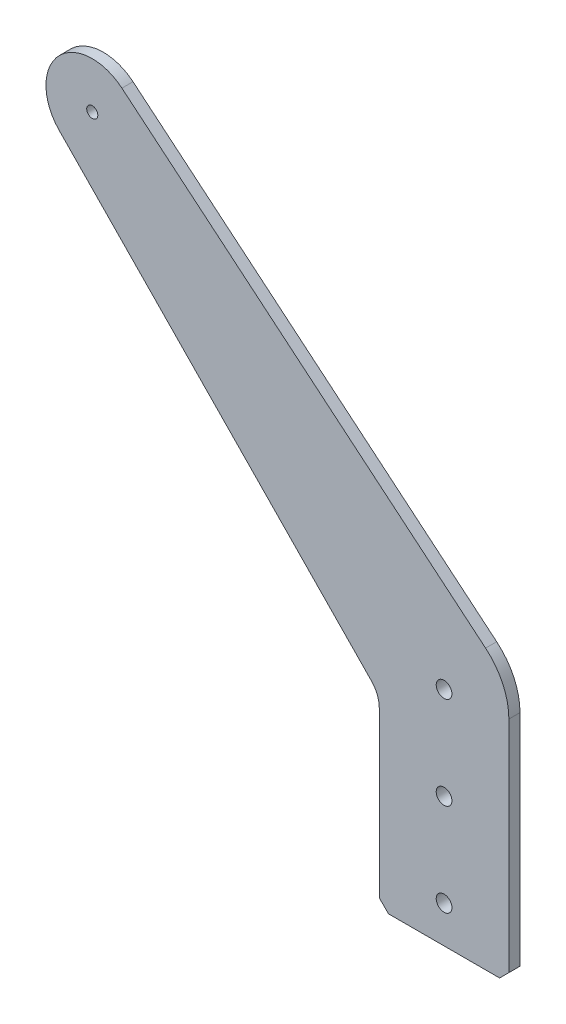
from build123d import *

# Parameters (mm, degrees)
SKETCH_1_R      = 3
SKETCH_1_R_2    = 4.25
EXTRUDE_1_DEPTH = 6
CHAMFER_1_SIZE  = 5


with BuildPart() as part:
    # 草图1 → 凸台-拉伸1 (new body)
    with BuildSketch(Plane.XY):
        with BuildLine():
            Line((16.006925776, 19.203601933), (212.409696086, -144.505507303))
            ThreePointArc((212.409696086, -144.505507303), (221.696524755, -156.547022178), (225, -171.390550009))
            Line((225, -171.390550009), (225, -295))
            Line((225, -295), (155, -295))
            Line((155, -295), (155, -201.097000919))
            ThreePointArc((155, -201.097000919), (153.895948255, -195.4487603), (150.746317055, -190.631979669))
            Line((150.746317055, -190.631979669), (-17.910528426, -17.441702082))
            ThreePointArc((-17.910528426, -17.441702082), (-18.347356822, 16.981592907), (16.006925776, 19.203601933))
        make_face()
        Circle(SKETCH_1_R, mode=Mode.SUBTRACT)
        with Locations((190, -275)):
            Circle(SKETCH_1_R_2, mode=Mode.SUBTRACT)
        with Locations((190, -225)):
            Circle(SKETCH_1_R_2, mode=Mode.SUBTRACT)
        with Locations((190, -175)):
            Circle(SKETCH_1_R_2, mode=Mode.SUBTRACT)
    extrude(amount=EXTRUDE_1_DEPTH)

    # 倒角1
    chamfer_1_edges = [part.edges().sort_by_distance(p)[0] for p in [
        (225, -295, 3),
        (155, -295, 3),
    ]]
    chamfer(chamfer_1_edges, length=CHAMFER_1_SIZE)


solid = part.part
